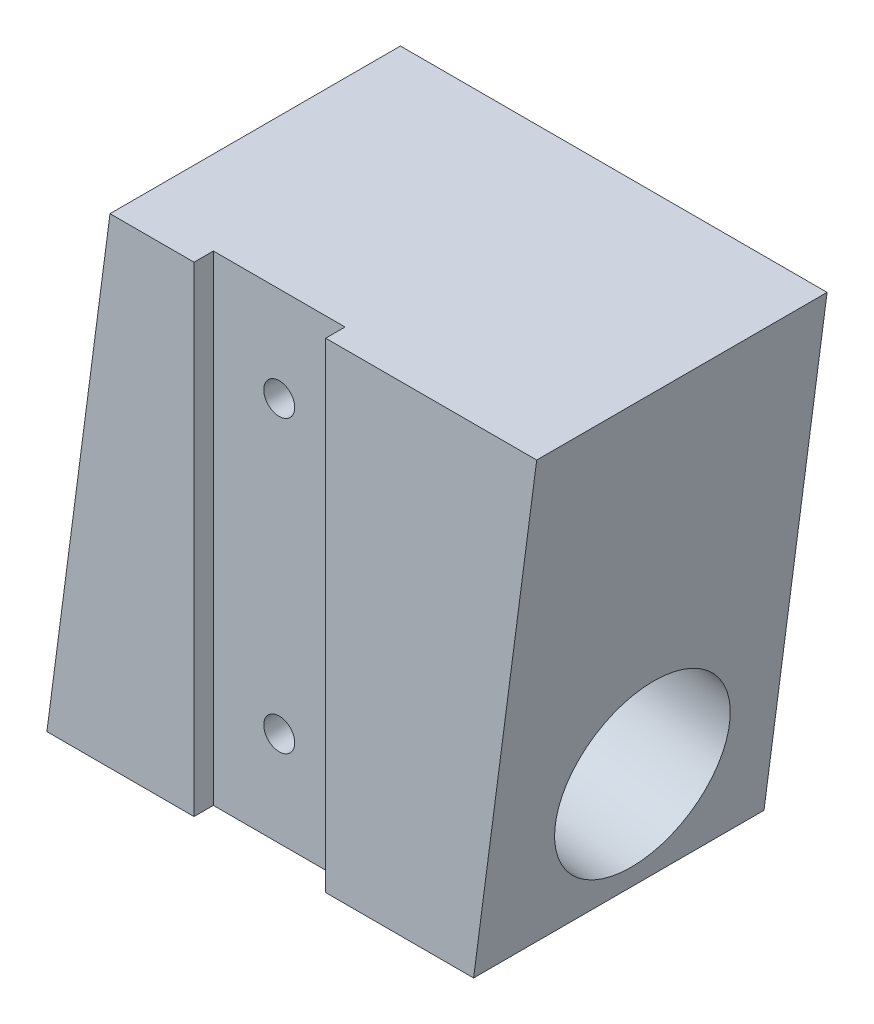
from build123d import *

# Parameters (mm, degrees)
SKETCH_1_W          = 25.3
SKETCH_1_H          = 24.8
EXTRUDE_1_DEPTH     = 15
CUT_EXTRUDE_1_REACH = 30.897
CUT_EXTRUDE_2_REACH = 37.009
SKETCH_3_W          = 6.8
SKETCH_3_H          = 1
CUT_EXTRUDE_3_REACH = 33.713
SKETCH_5_R          = 4.5
SKETCH_7_R          = 0.8
CUT_EXTRUDE_4_DEPTH = 6


with BuildPart() as part:
    # 草图1 → 凸台-拉伸1 (new body)
    with BuildSketch(Plane.XY):
        with Locations((-6.986164384, -2.581917808)):
            Rectangle(SKETCH_1_W, SKETCH_1_H)
    extrude(amount=EXTRUDE_1_DEPTH)

    # 草图2 → 切除-拉伸1 (cut, up to next)
    with BuildSketch(Plane(origin=(0, 0, 0), x_dir=(-1, 0, 0), z_dir=(0, 0, -1)), mode=Mode.PRIVATE) as cut_extrude_1_sk1:
        Polygon((-5.663835616, 9.818082192), (-2.403835616, -14.981917808), (-5.663835616, -14.981917808), align=None)
    cut_extrude_1_tool1 = extrude(cut_extrude_1_sk1.sketch, amount=-CUT_EXTRUDE_1_REACH, mode=Mode.PRIVATE) & part.part
    # 草图2 → 切除-拉伸1 (cut, up to next)
    with BuildSketch(Plane(origin=(0, 0, 0), x_dir=(-1, 0, 0), z_dir=(0, 0, -1)), mode=Mode.PRIVATE) as cut_extrude_1_sk2:
        Polygon((16.376164384, 9.818082192), (19.636164384, 9.818082192), (19.636164384, -14.981917808), align=None)
    cut_extrude_1_tool2 = extrude(cut_extrude_1_sk2.sketch, amount=-CUT_EXTRUDE_1_REACH, mode=Mode.PRIVATE) & part.part
    add(cut_extrude_1_tool1.solids().sort_by_distance((4.577169, -6.715251, 0))[0], mode=Mode.SUBTRACT)
    add(cut_extrude_1_tool2.solids().sort_by_distance((-18.549498, 1.551416, 0))[0], mode=Mode.SUBTRACT)

    # 草图3 → 切除-拉伸2 (cut, up to next)
    with BuildSketch(Plane.XZ.offset(14.981917808), mode=Mode.PRIVATE) as cut_extrude_2_sk1:
        with Locations((-8.636164384, 14.5)):
            Rectangle(SKETCH_3_W, SKETCH_3_H)
    cut_extrude_2_tool1 = extrude(cut_extrude_2_sk1.sketch, amount=-CUT_EXTRUDE_2_REACH, mode=Mode.PRIVATE) & part.part
    add(cut_extrude_2_tool1.solids().sort_by_distance((-8.636164, -14.981918, 14.5))[0], mode=Mode.SUBTRACT)

    # 草图5 → 切除-拉伸3 (cut, up to next)
    with BuildSketch(Plane(origin=(4.298949072, -0.565103789, 0), x_dir=(0, 0, -1), z_dir=(0.9914706167018176, -0.13033041171160964, 0)), mode=Mode.PRIVATE) as cut_extrude_3_sk1:
        with Locations(Location((-7, -9.013320677, 0), (0, 0, 90))):
            Circle(SKETCH_5_R)
    cut_extrude_3_tool1 = extrude(cut_extrude_3_sk1.sketch, amount=-CUT_EXTRUDE_3_REACH, mode=Mode.PRIVATE) & part.part
    add(cut_extrude_3_tool1.solids().sort_by_distance((3.124239, -9.501546, 7))[0], mode=Mode.SUBTRACT)

    # 草图7 → 切除-拉伸4 (cut)
    with BuildSketch(Plane.XY.offset(14)):
        with Locations((-8.636164384, 4.918082192)):
            Circle(SKETCH_7_R)
        with Locations((-8.636164384, -10.081917808)):
            Circle(SKETCH_7_R)
    extrude(amount=-CUT_EXTRUDE_4_DEPTH, mode=Mode.SUBTRACT)


solid = part.part
